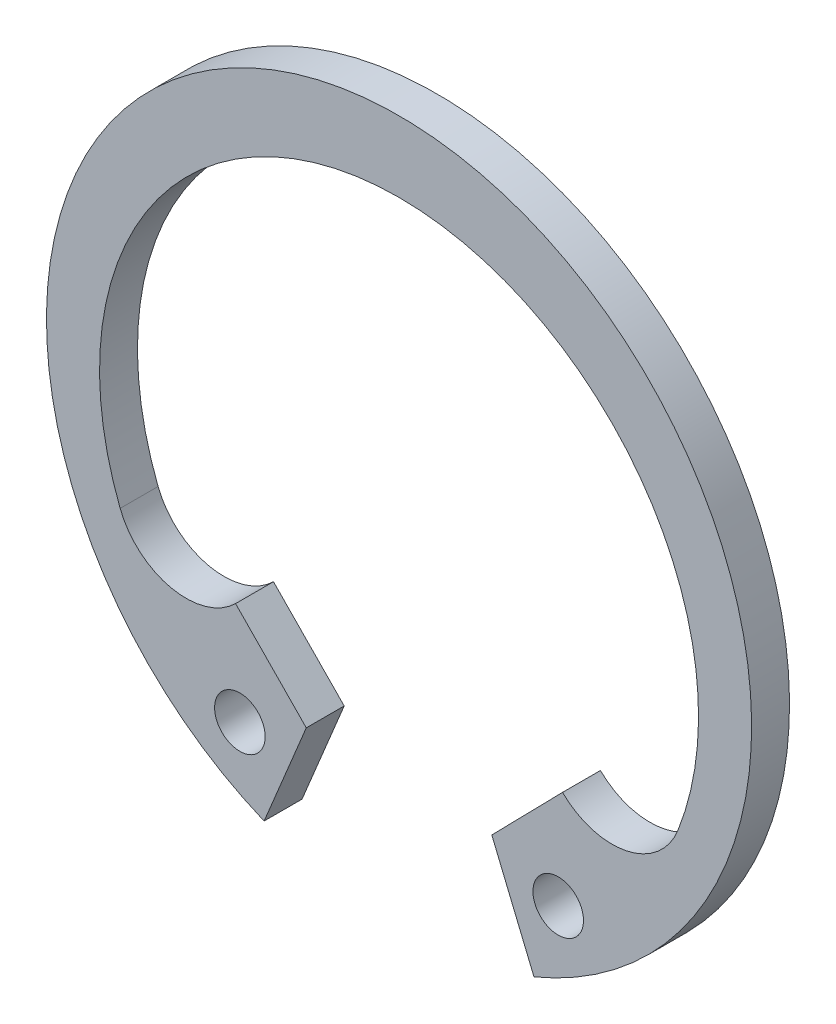
from build123d import *

# Parameters (mm, degrees)
SKETCH_1_R        = 1
EXTRUDE_952_DEPTH = 1.5


with BuildPart() as part:
    # 草图1 → Extrude 952 (new body)
    with BuildSketch(Plane.XY):
        with BuildLine():
            Line((-6.468002299, -6.001541065), (-3.669934116, -8.860004717))
            Line((-3.669934116, -8.860004717), (-5.338433881, -12.888119479))
            ThreePointArc((-5.338433881, -12.888119479), (0, 13.95), (5.338433881, -12.888119479))
            Line((5.338433881, -12.888119479), (3.669934116, -8.860004717))
            Line((3.669934116, -8.860004717), (6.468002299, -6.001541065))
            ThreePointArc((6.468002299, -6.001541065), (9.014108926, -6.738296556), (11.033790366, -5.021801727))
            ThreePointArc((11.033790366, -5.021801727), (0, 11.15), (-11.033790366, -5.021801727))
            ThreePointArc((-11.033790366, -5.021801727), (-9.014108926, -6.738296556), (-6.468002299, -6.001541065))
        make_face()
        with Locations((-6.298089329, -9.978680815)):
            Circle(SKETCH_1_R, mode=Mode.SUBTRACT)
        with Locations(Location((6.298089329, -9.978680815, 0), (0, 0, 180))):
            Circle(SKETCH_1_R, mode=Mode.SUBTRACT)
    extrude(amount=EXTRUDE_952_DEPTH)


solid = part.part
